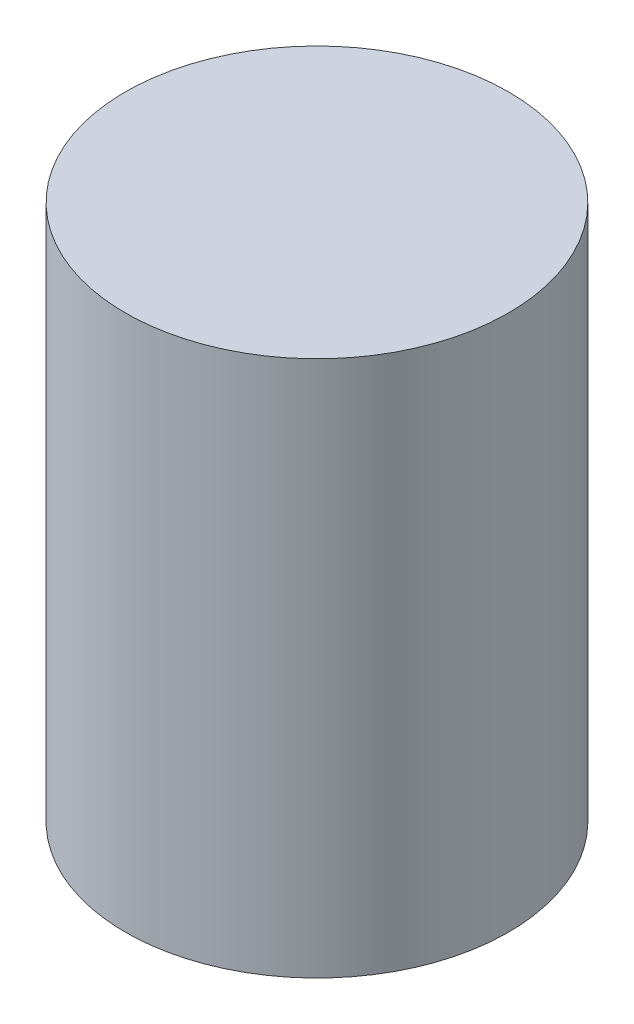
SolidWorks part; units mm, degrees
ref_plane "前视基准面" through (0, 0, 0) normal (0, 0, 1) x (1, 0, 0)
ref_plane "上视基准面" through (0, 0, 0) normal (0, 1, 0) x (1, 0, 0)
ref_plane "右视基准面" through (0, 0, 0) normal (1, 0, 0) x (0, 0, -1)
sketch "草图1" plane through (0, 0, 0) normal (0, 0, 1) x (1, 0, 0)
  line L1 (0, 0) -> (-12.5, 0)
  line L2 (0, 0) -> (0, 35)
  line L3 (0, 35) -> (-12.5, 35)
  line L4 (-12.5, 0) -> (-12.5, 35)
  dimension "D1" = 12.5
  dimension "D2" = 35
revolve "旋转1" add sketch "草图1" angle 360 about L2
equation "\"图号代码1\"= \"图号代码\""
equation "\"名称代码2\"= \"名称代码\""
